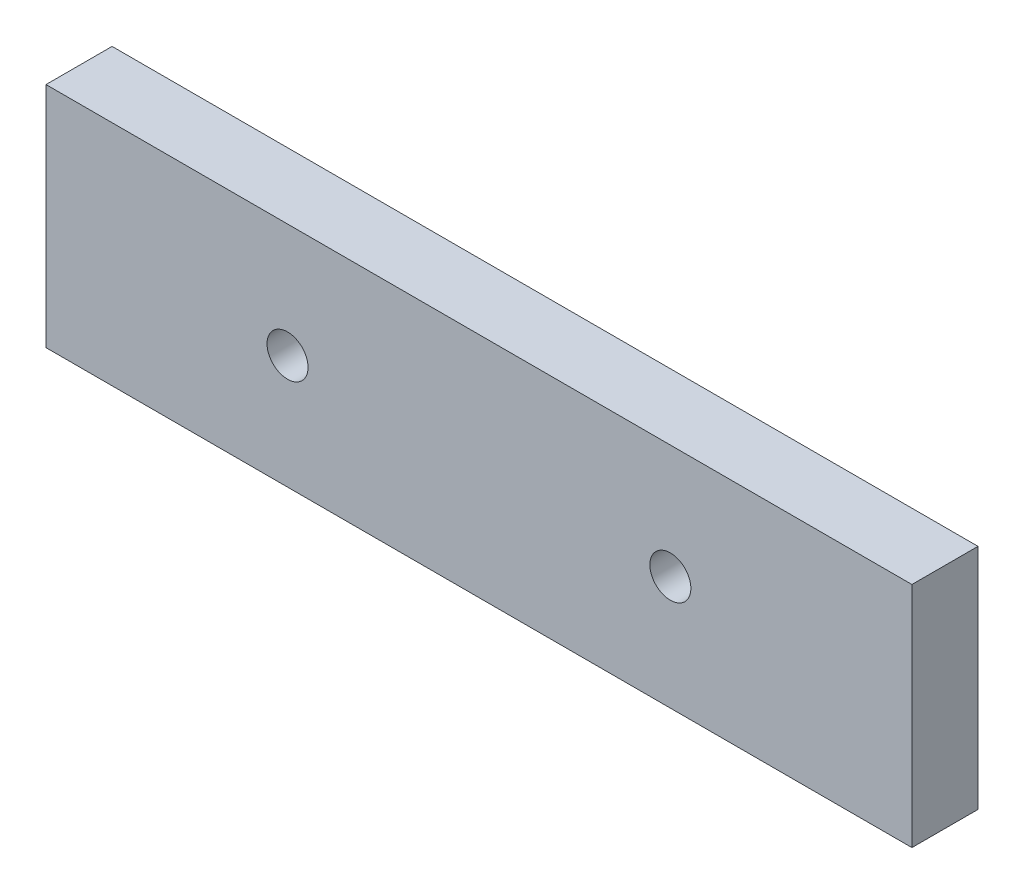
from build123d import *

# Parameters (mm, degrees)
SKETCH_1_W      = 190
SKETCH_1_H      = 50
SKETCH_1_R      = 4.5
EXTRUDE_1_DEPTH = 7.25


with BuildPart() as part:
    # 草图1 → 凸台-拉伸1 (new, symmetric)
    with BuildSketch(Plane.XY):
        Rectangle(SKETCH_1_W, SKETCH_1_H)
        with Locations(Location((-42, 0, 0), (0, 0, 180))):
            Circle(SKETCH_1_R, mode=Mode.SUBTRACT)
        with Locations(Location((42, 0, 0), (0, 0, 180))):
            Circle(SKETCH_1_R, mode=Mode.SUBTRACT)
    extrude(amount=EXTRUDE_1_DEPTH, both=True)


solid = part.part
